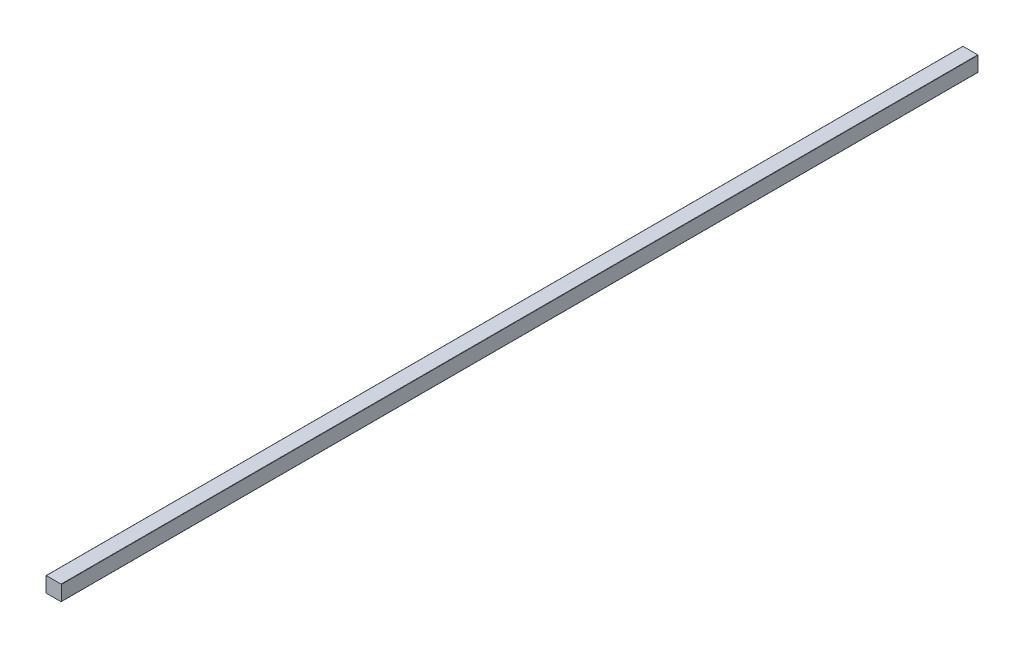
SolidWorks part; units mm, degrees
material "Plain carbon steel"
ref_plane "Front Plane" through (0, 0, 0) normal (0, 0, 1) x (1, 0, 0)
ref_plane "Top Plane" through (0, 0, 0) normal (0, 1, 0) x (1, 0, 0)
ref_plane "Right Plane" through (0, 0, 0) normal (1, 0, 0) x (0, 0, -1)
sketch "Sketch1" plane through (0, 0, 0) normal (0, 0, 1) x (1, 0, 0)
  line L1 (-11.5, -12) -> (11.5, -12)
  line L2 (-12, -11.5) -> (-12, 11.5)
  line L3 (-11.5, 12) -> (11.5, 12)
  line L4 (12, -11.5) -> (12, 11.5)
  line L5 (-12, -12) -> (12, 12) construction
  line L6 (-12, 12) -> (12, -12) construction
  arc A0 (-12, 11.5) -> (-11.5, 12) centre (-11.5, 11.5) cw
  arc A1 (-11.5, -12) -> (-12, -11.5) centre (-11.5, -11.5) cw
  arc A2 (11.5, -12) -> (12, -11.5) centre (11.5, -11.5) ccw
  arc A3 (11.5, 12) -> (12, 11.5) centre (11.5, 11.5) cw
  point P0 (0, 0)
  dimension "D2" = 0.5
  dimension "D1" = 24
extrude "Boss-Extrude1" add sketch "Sketch1" along normal mid plane 1440
